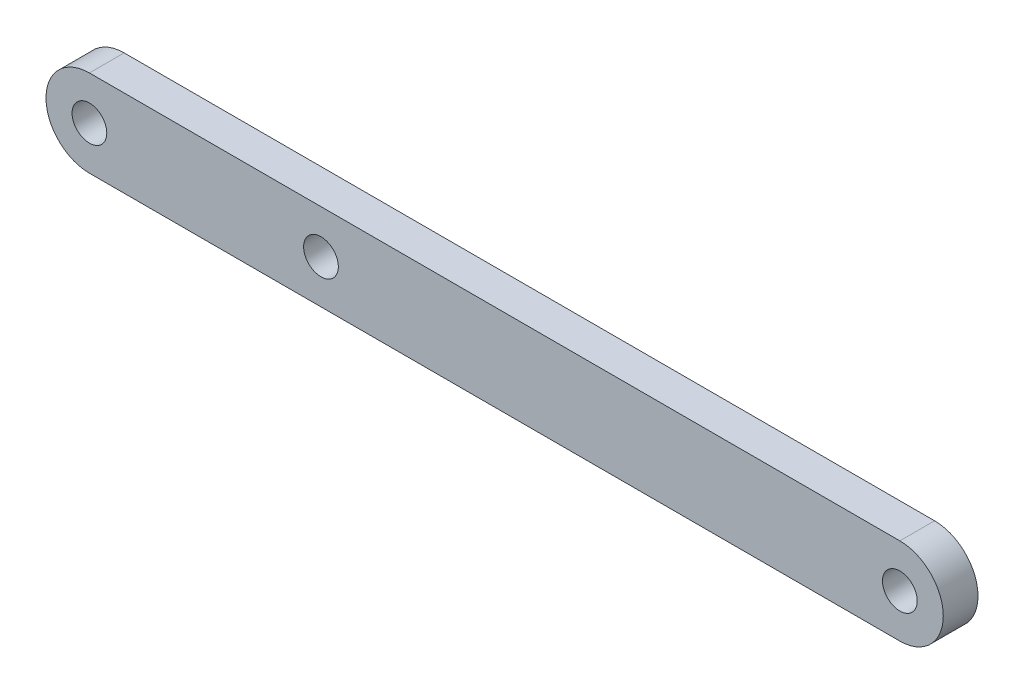
from build123d import *

# Parameters (mm, degrees)
SKETCH1_R           = 3
BOSS_EXTRUDE1_DEPTH = 6


with BuildPart() as part:
    # Sketch1 → Boss-Extrude1 (new body)
    with BuildSketch(Plane.XY):
        with BuildLine():
            Line((0, 7.5), (140, 7.5))
            ThreePointArc((140, 7.5), (147.5, 0), (140, -7.5))
            Line((140, -7.5), (0, -7.5))
            ThreePointArc((0, -7.5), (-7.5, 0), (0, 7.5))
        make_face()
        Circle(SKETCH1_R, mode=Mode.SUBTRACT)
        with Locations((40, 0)):
            Circle(SKETCH1_R, mode=Mode.SUBTRACT)
        with Locations((140, 0)):
            Circle(SKETCH1_R, mode=Mode.SUBTRACT)
    extrude(amount=BOSS_EXTRUDE1_DEPTH)


solid = part.part
